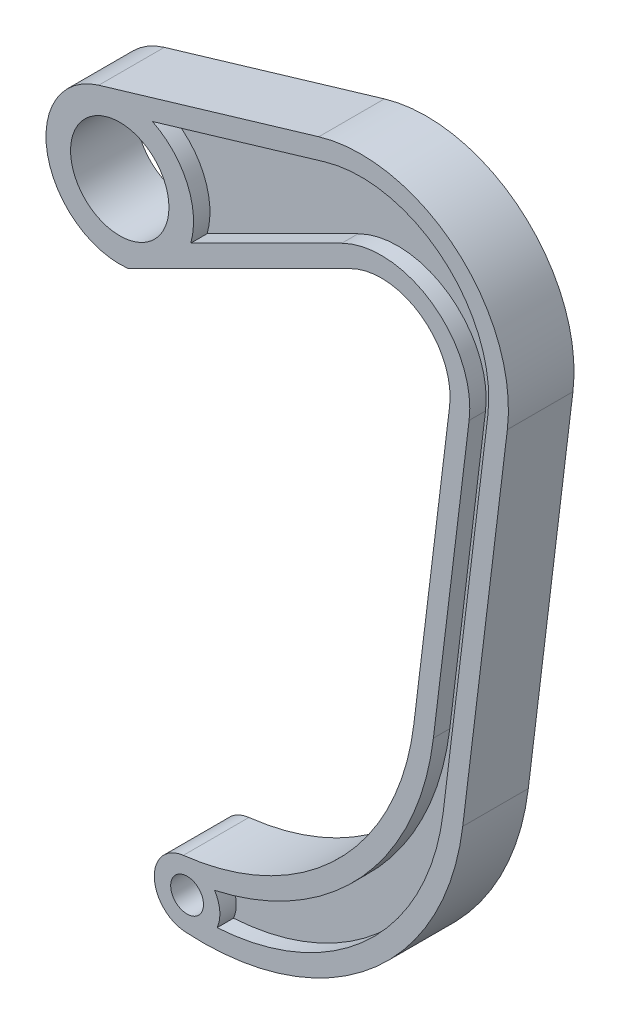
SolidWorks part; units mm, degrees
ref_plane "Front Plane" through (0, 0, 0) normal (0, 0, 1) x (1, 0, 0)
ref_plane "Top Plane" through (0, 0, 0) normal (0, 1, 0) x (1, 0, 0)
ref_plane "Right Plane" through (0, 0, 0) normal (1, 0, 0) x (0, 0, -1)
sketch "Sketch2" plane through (0, 0, 0) normal (0, 0, 1) x (1, 0, 0)
  line L4 (618.0999, 106.5178) -> (565.6628, 90.9369)
  line L5 (577.354, 64.655) -> (623.4063, 87.6645)
  line L6 (662.2235, 60.2805) -> (651.331, -29.0579)
  line L7 (654.3166, -47.1719) -> (667.9215, 64.4132)
  line L8 (618.0999, 106.5178) -> (565.6628, 90.9369)
  line L9 (577.354, 64.655) -> (623.4063, 87.6645)
  line L10 (662.2235, 60.2805) -> (651.331, -29.0579)
  line L11 (654.3166, -47.1719) -> (667.9215, 64.4132)
  arc A6 (577.354, 64.655) -> (565.6628, 90.9369) centre (555.6991, 70.7633) ccw
  arc A7 (662.2235, 60.2805) -> (623.4063, 87.6645) centre (635.4579, 63.5439) ccw
  arc A8 (584.6064, -102.6044) -> (651.331, -29.0579) centre (565.9631, -18.6495) ccw
  arc A9 (585.3858, -112.0773) -> (584.6064, -102.6044) centre (576.2272, -108.0623) ccw
  arc A10 (585.3858, -112.0773) -> (654.3166, -47.1719) centre (580.8606, -38.2158) ccw
  arc A11 (667.9215, 64.4132) -> (618.0999, 106.5178) centre (629.2082, 69.1332) ccw
  arc A12 (577.354, 64.655) -> (565.6628, 90.9369) centre (555.6991, 70.7633) ccw
  arc A13 (662.2235, 60.2805) -> (623.4063, 87.6645) centre (635.4579, 63.5439) ccw
  arc A14 (584.6064, -102.6044) -> (651.331, -29.0579) centre (565.9631, -18.6495) ccw
  arc A15 (585.3858, -112.0773) -> (584.6064, -102.6044) centre (576.2272, -108.0623) ccw
  arc A16 (585.3858, -112.0773) -> (654.3166, -47.1719) centre (580.8606, -38.2158) ccw
  arc A17 (667.9215, 64.4132) -> (618.0999, 106.5178) centre (629.2082, 69.1332) ccw
  dimension "D1" = 0
extrude "Boss-Extrude1" add sketch "Sketch2" against normal up to surface (10 mm away)
sketch "Sketch3" plane through (0, 0, 5) normal (0, 0, 1) x (1, 0, 0)
  line L4 (558.2651, 48.4101) -> (626.088, 82.2972)
  line L5 (656.2676, 61.0067) -> (645.3751, -28.3317)
  line L6 (660.2725, -47.898) -> (673.8774, 63.687)
  line L7 (616.3909, 112.2693) -> (549.2904, 92.3313)
  line L8 (558.2651, 48.4101) -> (626.088, 82.2972)
  line L9 (656.2676, 61.0067) -> (645.3751, -28.3317)
  line L10 (660.2725, -47.898) -> (673.8774, 63.687)
  line L11 (616.3909, 112.2693) -> (549.2904, 92.3313)
  line L12 (618.0999, 106.5178) -> (565.6628, 90.9369)
  line L13 (577.354, 64.655) -> (623.4063, 87.6645)
  line L14 (662.2235, 60.2805) -> (651.331, -29.0579)
  line L15 (654.3166, -47.1719) -> (667.9215, 64.4132)
  line L16 (618.0999, 106.5178) -> (565.6628, 90.9369)
  line L17 (577.354, 64.655) -> (623.4063, 87.6645)
  line L18 (662.2235, 60.2805) -> (651.331, -29.0579)
  line L19 (654.3166, -47.1719) -> (667.9215, 64.4132)
  arc A0 (553.9884, 85.6654) -> (557.4097, 55.8612) centre (555.6991, 70.7633) ccw construction
  arc A1 (557.4097, 55.8612) -> (553.9884, 85.6654) centre (555.6991, 70.7633) ccw construction
  arc A2 (553.9884, 85.6654) -> (557.4097, 55.8612) centre (555.6991, 70.7633) ccw
  arc A3 (557.4097, 55.8612) -> (553.9884, 85.6654) centre (555.6991, 70.7633) ccw
  arc A6 (549.2904, 92.3313) -> (558.2651, 48.4101) centre (555.6991, 70.7633) ccw
  arc A7 (656.2676, 61.0067) -> (626.088, 82.2972) centre (635.4579, 63.5439) ccw
  arc A8 (575.0868, -98.1275) -> (645.3751, -28.3317) centre (565.9631, -18.6495) ccw
  arc A9 (575.0868, -98.1275) -> (575.5653, -118.0404) centre (576.2272, -108.0623) ccw
  arc A10 (575.5653, -118.0404) -> (660.2725, -47.898) centre (580.8606, -38.2158) ccw
  arc A11 (673.8774, 63.687) -> (616.3909, 112.2693) centre (629.2082, 69.1332) ccw
  arc A12 (549.2904, 92.3313) -> (558.2651, 48.4101) centre (555.6991, 70.7633) ccw
  arc A13 (656.2676, 61.0067) -> (626.088, 82.2972) centre (635.4579, 63.5439) ccw
  arc A14 (575.0868, -98.1275) -> (645.3751, -28.3317) centre (565.9631, -18.6495) ccw
  arc A15 (575.0868, -98.1275) -> (575.5653, -118.0404) centre (576.2272, -108.0623) ccw
  arc A16 (575.5653, -118.0404) -> (660.2725, -47.898) centre (580.8606, -38.2158) ccw
  arc A17 (673.8774, 63.687) -> (616.3909, 112.2693) centre (629.2082, 69.1332) ccw
  arc A18 (667.9215, 64.4132) -> (618.0999, 106.5178) centre (629.2082, 69.1332) ccw
  arc A19 (577.354, 64.655) -> (565.6628, 90.9369) centre (555.6991, 70.7633) ccw
  arc A20 (662.2235, 60.2805) -> (623.4063, 87.6645) centre (635.4579, 63.5439) ccw
  arc A21 (584.6064, -102.6044) -> (651.331, -29.0579) centre (565.9631, -18.6495) ccw
  arc A22 (585.3858, -112.0773) -> (584.6064, -102.6044) centre (576.2272, -108.0623) ccw
  arc A23 (585.3858, -112.0773) -> (654.3166, -47.1719) centre (580.8606, -38.2158) ccw
  arc A24 (667.9215, 64.4132) -> (618.0999, 106.5178) centre (629.2082, 69.1332) ccw
  arc A25 (577.354, 64.655) -> (565.6628, 90.9369) centre (555.6991, 70.7633) ccw
  arc A26 (662.2235, 60.2805) -> (623.4063, 87.6645) centre (635.4579, 63.5439) ccw
  arc A27 (584.6064, -102.6044) -> (651.331, -29.0579) centre (565.9631, -18.6495) ccw
  arc A28 (585.3858, -112.0773) -> (584.6064, -102.6044) centre (576.2272, -108.0623) ccw
  arc A29 (585.3858, -112.0773) -> (654.3166, -47.1719) centre (580.8606, -38.2158) ccw
  arc M21 (575.657, -103.0949) -> (576.7974, -113.0297) centre (576.2272, -108.0623) cw
  arc M22 (576.7974, -113.0297) -> (575.657, -103.0949) centre (576.2272, -108.0623) cw
  arc M23 (553.9884, 85.6654) -> (557.4097, 55.8612) centre (555.6991, 70.7633) cw
  arc M24 (557.4097, 55.8612) -> (553.9884, 85.6654) centre (555.6991, 70.7633) cw
  line M25 (667.9215, 64.4132) -> (654.3166, -47.1719)
  arc M26 (654.3166, -47.1719) -> (585.3858, -112.0773) centre (580.8606, -38.2158) cw
  arc M27 (585.3858, -112.0773) -> (584.6064, -102.6044) centre (576.2272, -108.0623) ccw
  arc M28 (584.6064, -102.6044) -> (651.331, -29.0579) centre (565.9631, -18.6495) ccw
  line M29 (651.331, -29.0579) -> (662.2235, 60.2805)
  arc M30 (662.2235, 60.2805) -> (623.4063, 87.6645) centre (635.4579, 63.5439) ccw
  line M31 (623.4063, 87.6645) -> (577.354, 64.655)
  arc M32 (577.354, 64.655) -> (565.6628, 90.9369) centre (555.6991, 70.7633) ccw
  line M33 (565.6628, 90.9369) -> (618.0999, 106.5178)
  arc M34 (618.0999, 106.5178) -> (667.9215, 64.4132) centre (629.2082, 69.1332) cw
  arc M35 (549.2904, 92.3313) -> (558.2651, 48.4101) centre (555.6991, 70.7633) ccw
  line M36 (558.2651, 48.4101) -> (626.088, 82.2972)
  arc M37 (626.088, 82.2972) -> (656.2676, 61.0067) centre (635.4579, 63.5439) cw
  line M38 (656.2676, 61.0067) -> (645.3751, -28.3317)
  arc M39 (645.3751, -28.3317) -> (575.0868, -98.1275) centre (565.9631, -18.6495) cw
  arc M40 (575.0868, -98.1275) -> (575.5653, -118.0404) centre (576.2272, -108.0623) ccw
  arc M41 (575.5653, -118.0404) -> (660.2725, -47.898) centre (580.8606, -38.2158) ccw
  line M42 (660.2725, -47.898) -> (673.8774, 63.687)
  arc M43 (673.8774, 63.687) -> (616.3909, 112.2693) centre (629.2082, 69.1332) ccw
  line M44 (616.3909, 112.2693) -> (549.2904, 92.3313)
  dimension "D1" = 0
  dimension "D2" = 0
extrude "Boss-Extrude2" add sketch "Sketch3" against normal up to surface (20 mm away) contours M44 M35 M36 M37 M38 M39 M40 M41 M42 M43 M34 M25 M26 M27 M28 M29 M30 M31 M32 M33 M24 M23 M22 M21
